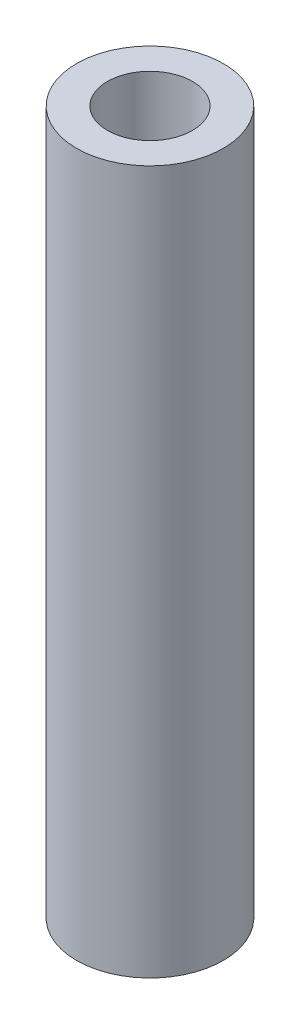
from build123d import *

# Parameters (mm, degrees)
SKETCH_1_R          = 9.5
EXTRUDE_1_DEPTH     = 91
SKETCH_2_R          = 5.5
CUT_EXTRUDE_1_DEPTH = 75
HOLE_WIZARD_M6_1_D  = 5


with BuildPart() as part:
    # 草图1 → 凸台-拉伸1 (new body)
    with BuildSketch(Plane(origin=(0, 0, 0), x_dir=(1, 0, 0), z_dir=(0, 1, 0))):
        with Locations(Location((0, 0, 0), (0, 0, 270))):
            Circle(SKETCH_1_R)
    extrude(amount=EXTRUDE_1_DEPTH)

    # 草图2 → 切除-拉伸1 (cut)
    with BuildSketch(Plane(origin=(0, 91, 0), x_dir=(1, 0, 0), z_dir=(0, 1, 0))):
        with Locations(Location((0, 0, 0), (0, 0, 270))):
            Circle(SKETCH_2_R)
    extrude(amount=-CUT_EXTRUDE_1_DEPTH, mode=Mode.SUBTRACT)

    # M6 螺纹孔1 (through all)
    with Locations(Plane.XZ):
        with Locations((0, 0)):
            Hole(HOLE_WIZARD_M6_1_D / 2)


solid = part.part
